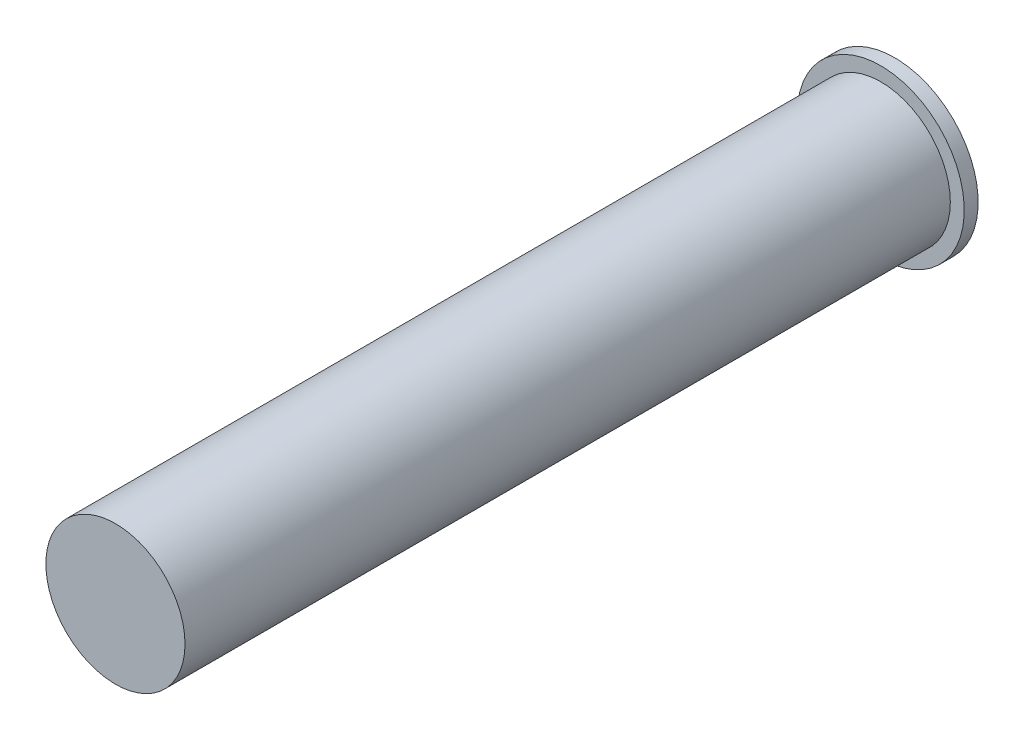
from build123d import *

# Parameters (mm, degrees)
SKETCH_1_R      = 5
EXTRUDE_1_DEPTH = 55
SKETCH_2_R      = 6
EXTRUDE_2_DEPTH = 1


with BuildPart() as part:
    # 草图1 → 凸台-拉伸1 (new body)
    with BuildSketch(Plane.XY):
        Circle(SKETCH_1_R)
    extrude(amount=EXTRUDE_1_DEPTH)

    # 草图2 → 凸台-拉伸2 (add)
    with BuildSketch(Plane(origin=(0, 0, 0), x_dir=(-1, 0, 0), z_dir=(0, 0, -1))):
        Circle(SKETCH_2_R)
    extrude(amount=EXTRUDE_2_DEPTH)


solid = part.part
